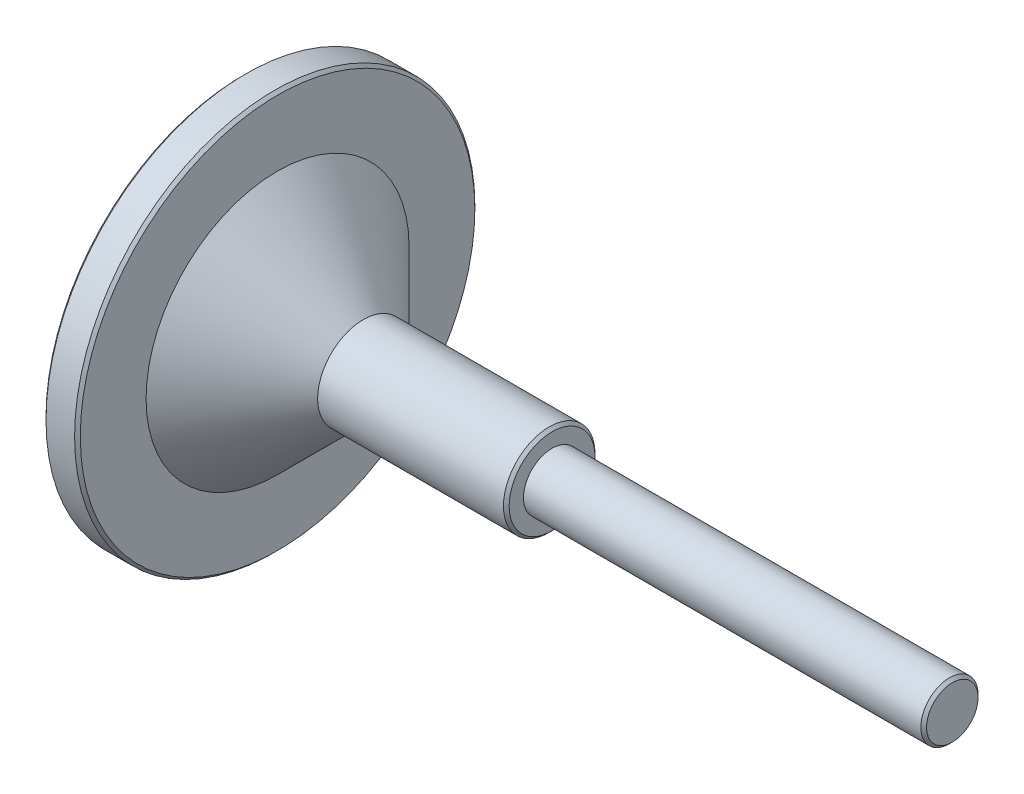
SolidWorks part; units mm, degrees
material "45(Ni)"
ref_plane "Front Plane" through (0, 0, 0) normal (0, 0, 1) x (1, 0, 0)
ref_plane "Top Plane" through (0, 0, 0) normal (0, 1, 0) x (1, 0, 0)
ref_plane "Right Plane" through (0, 0, 0) normal (1, 0, 0) x (0, 0, -1)
sketch "Sketch1" plane through (0, 0, 0) normal (0, 0, 1) x (1, 0, 0)
  line L0 (0, 0) -> (296.6277, 0) construction
  line L1 (0, 0) -> (0, 35)
  line L2 (0, 35) -> (6, 35)
  line L3 (6, 35) -> (6, 8)
  line L4 (6, 8) -> (54, 8)
  line L5 (54, 8) -> (54, 5)
  line L6 (54, 5) -> (124, 5)
  line L7 (124, 5) -> (124, 0)
  line L8 (124, 0) -> (0, 0)
  dimension "D1" = 70
  dimension "D2" = 16
  dimension "D3" = 10
  dimension "D4" = 6
  dimension "D5" = 48
  dimension "D6" = 70
revolve "Revolve1" add sketch "Sketch1" angle 360 about L0
cosmetic thread "Cosmetic Thread1" parameters "D1"=20, "D2"=9
chamfer "Chamfer1" distance 0.5 angle 45 3 edges at (54, 0, 8) (6, 0, 35) (0, 0, 35)
chamfer "Chamfer2" distance 0.5 angle 45 1 edges at (124, 0, 5)
chamfer "Chamfer3" distance 15 angle 45 1 edges at (6, 0, 8)
